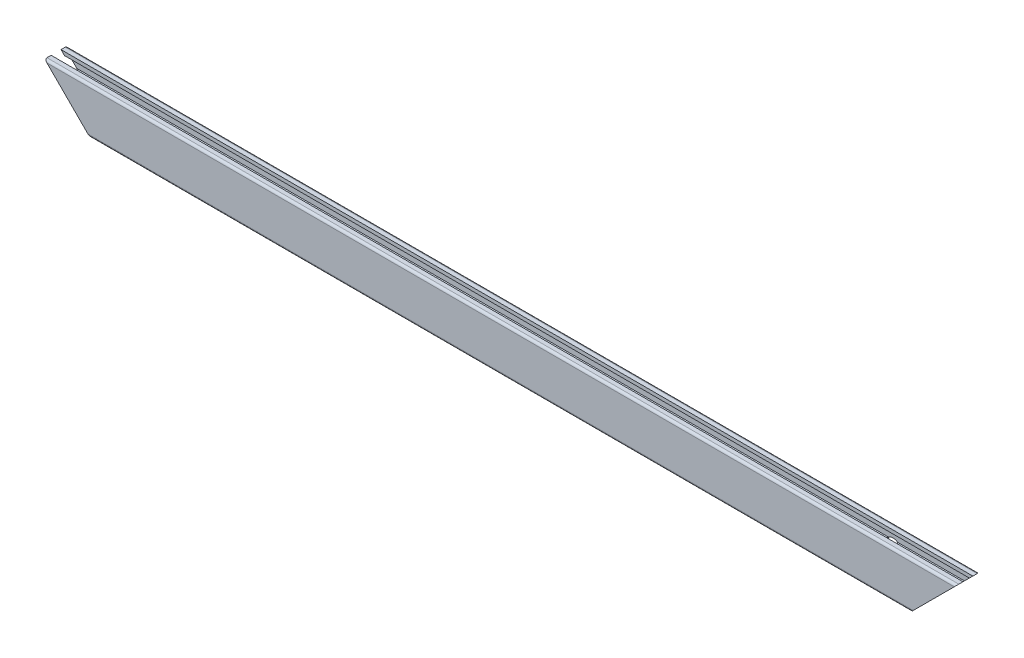
SolidWorks part; units mm, degrees
ref_plane "前视" through (0, 0, 0) normal (0, 0, 1) x (1, 0, 0)
ref_plane "上视" through (0, 0, 0) normal (0, 1, 0) x (1, 0, 0)
ref_plane "右视" through (0, 0, 0) normal (1, 0, 0) x (0, 0, -1)
sketch3d "3D草图1"
  line L0 (-300, 0, 0) -> (300, 0, 0)
  dimension "D1" = 600
other "结构构件1"
ref_plane "基准面1" through (-300, 0, 0) normal (1, 0, 0) x (0, 0, -1)
sketch "Sketch12" plane through (-300, 0, 0) normal (1, 0, 0) x (0, 0, -1)
  line L1 (0, 16.311) -> (0, -16.311) construction
  line L2 (0, 0) -> (9.513, 0) construction
  line L3 (-6, -15) -> (-3.25, -15)
  line L4 (-7.5, -13.5) -> (-7.5, 13.5)
  line L5 (-6, 15) -> (-3.25, 15)
  line L6 (7.5, -13.5) -> (7.5, 13.5)
  line L17 (3.25, 15) -> (6, 15)
  line L20 (-5.7, 12.7) -> (-5.7, 7)
  line L21 (-3.25, 12.7) -> (-5.7, 12.7)
  line L24 (5.7, 12.7) -> (5.7, 7)
  line L25 (3.25, 12.7) -> (5.7, 12.7)
  line L26 (-3.25, 15) -> (-3.25, 12.7)
  line L27 (3.25, 15) -> (3.25, 12.7)
  line L40 (5.7, -12.7) -> (5.7, -7)
  line L41 (3.25, -12.7) -> (5.7, -12.7)
  line L44 (-5.7, -12.7) -> (-5.7, -7)
  line L45 (-3.25, -12.7) -> (-5.7, -12.7)
  line L47 (3.25, -15) -> (3.25, -12.7)
  line L48 (-3.25, -15) -> (-3.25, -12.7)
  line L49 (3.25, -15) -> (6, -15)
  arc A0 (-6, -15) -> (-7.5, -13.5) centre (-6, -13.5) cw
  arc A1 (6, -15) -> (7.5, -13.5) centre (6, -13.5) ccw
  arc A2 (6, 15) -> (7.5, 13.5) centre (6, 13.5) cw
  arc A3 (-7.5, 13.5) -> (-6, 15) centre (-6, 13.5) cw
  circle A4 centre (0, 0) radius 2.5
  arc A5 (-5.7, 7) -> (5.7, 7) centre (0, 12.248) ccw
  arc A6 (-5.7, -7) -> (5.7, -7) centre (0, -12.248) cw
  point P4 (0, 0)
  point P21 (0, 0)
  point P44 (-7.5, 15)
  point P45 (7.5, 15)
  point P46 (7.5, -15)
  point P47 (-7.5, -15)
  point P48 (0, -15)
  point P49 (0, 15)
  dimension "D1" = 30
  dimension "D2" = 15
  dimension "D3" = 1.5
  dimension "D4" = 5
  dimension "D5" = 6.5
  dimension "D6" = 10.5
  dimension "D7" = 8
  dimension "D8" = 11.4
  dimension "D9" = 2.3
sketch "草图4" plane through (0, 0, 7.5) normal (0, 0, 1) x (1, 0, 0)
  line L0 (-300, 15) -> (-270, -15)
  line L2 (0, 0) -> (0, -85.0329) construction
  line L3 (-270, -15) -> (-300, -15)
  line L4 (-300, -15) -> (-300, 15)
  line L5 (300, -15) -> (300, 15)
  line L6 (270, -15) -> (300, -15)
  line L7 (300, 15) -> (270, -15)
  line L8 (300, 15) -> (-300, 15) construction
  line L9 (300, -15) -> (-300, -15) construction
  line L10 (-300, 13.5) -> (-300, -13.5) construction
extrude "切除-拉伸1" cut sketch "草图4" against normal through all
sketch "草图7" plane through (0, 0, -7.5) normal (0, 0, 1) x (1, 0, 0)
  line L0 (300, 15) -> (-300, 15) construction
  circle A0 centre (245, 3) radius 5
  dimension "D1" = 10
  dimension "D2" = 55
  dimension "D3" = 12
extrude "切除-拉伸2" cut sketch "草图7" along normal blind 4.999
